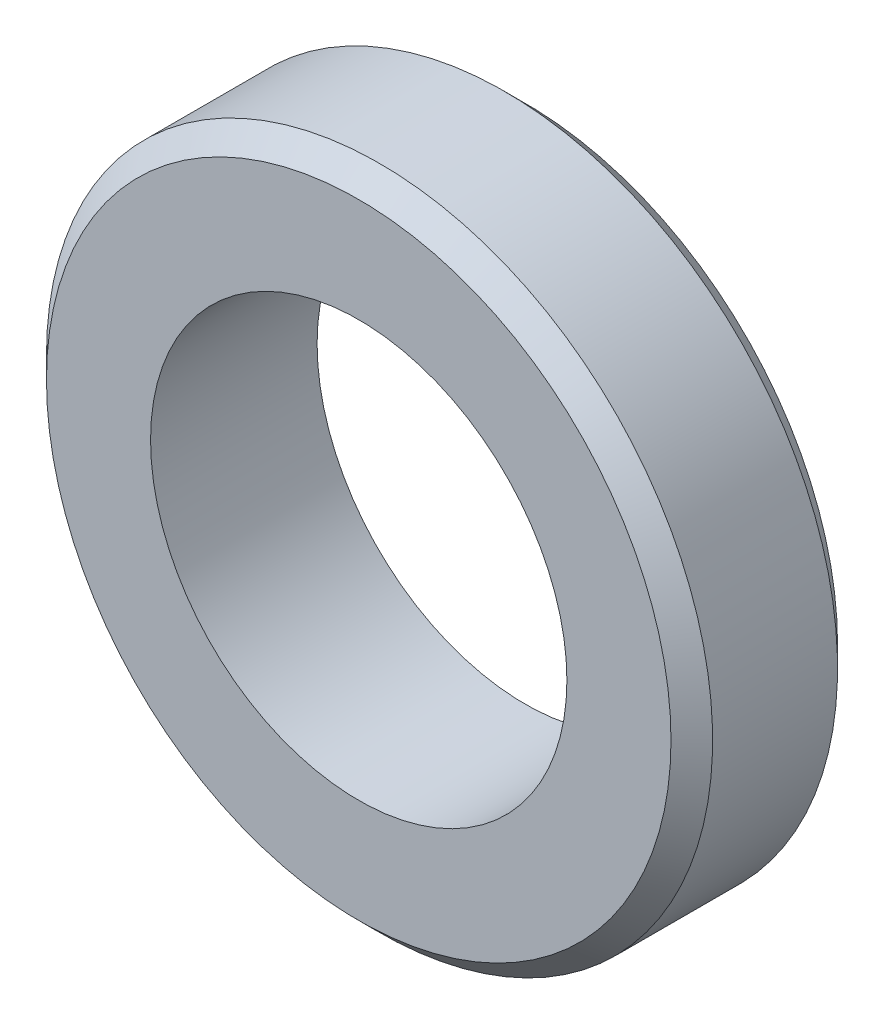
from build123d import *


with BuildPart() as part:
    # Sketch1 → Revolve1 (revolve)
    with BuildSketch(Plane.XZ, mode=Mode.PRIVATE) as revolve1_sk:
        Polygon((5, 4), (5, 0), (7.5, 0), (8, 0.5), (8, 3.5), (7.5, 4), align=None)
    revolve(revolve1_sk.sketch.rotate(Axis((0, 0, 4), (0, 0, -1)), 180), axis=Axis((0, 0, 4), (0, 0, -1)))


solid = part.part
